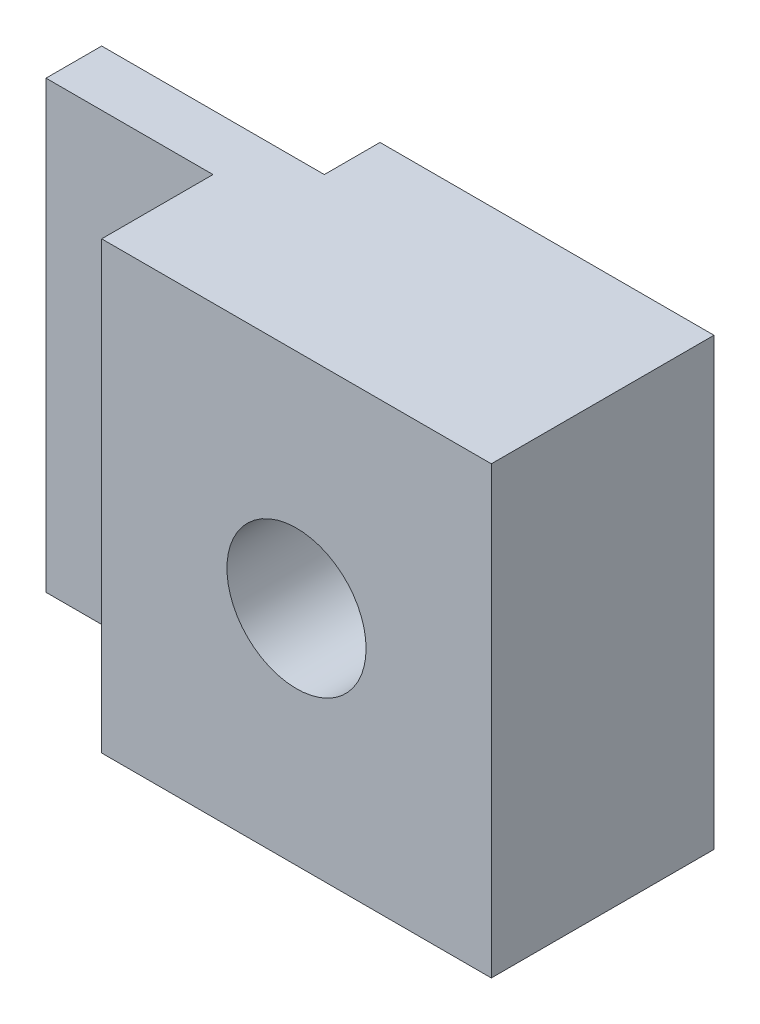
from build123d import *

# Parameters (mm, degrees)
SKETCH1_W             = 12
SKETCH1_H             = 8
BOSS_EXTRUDE1_DEPTH   = 2
SKETCH2_W             = 7
SKETCH2_H             = 8
BOSS_EXTRUDE2_DEPTH   = 2
SKETCH3_R             = 1.25
CUT_EXTRUDE1_DEPTH    = 10
CUT_EXTRUDE2_DEPTH    = 1
SKETCH5_W             = 2
SKETCH5_H             = 8
CUT_EXTRUDE3_DEPTH    = 7
MOVE_FACE1_BY         = 0.5
M3_TAPPED_HOLE4_D     = 2.5
M3_TAPPED_HOLE4_DEPTH = 7.5
M3_TAPPED_HOLE4_TIP   = 0.751075774


with BuildPart() as part:
    # Sketch1 → Boss-Extrude1 (new body)
    with BuildSketch(Plane.XY):
        with Locations((6, -4)):
            Rectangle(SKETCH1_W, SKETCH1_H)
    extrude(amount=BOSS_EXTRUDE1_DEPTH)

    # Sketch2 → Boss-Extrude2 (add)
    with BuildSketch(Plane.XY.offset(2)):
        with Locations((8.5, -4)):
            Rectangle(SKETCH2_W, SKETCH2_H)
    extrude(amount=BOSS_EXTRUDE2_DEPTH)

    # Sketch3 → Cut-Extrude1 (cut)
    with BuildSketch(Plane.XY.offset(4)):
        with Locations((8.5, -4)):
            Circle(SKETCH3_R)
    extrude(amount=-CUT_EXTRUDE1_DEPTH, mode=Mode.SUBTRACT)

    # Sketch4 → Cut-Extrude2 (cut)
    with BuildSketch(Plane(origin=(0, 0, 0), x_dir=(-1, 0, 0), z_dir=(0, 0, -1))):
        Polygon((0, -4), (0, 1.17366925), (-6, 1.17366925), (-6, -4), (-6, -6.5), (0, -6.5), align=None)
    extrude(amount=-CUT_EXTRUDE2_DEPTH, mode=Mode.SUBTRACT)

    # Sketch5 → Cut-Extrude3 (cut)
    with BuildSketch(Plane(origin=(0, 0, 0), x_dir=(-1, 0, 0), z_dir=(0, 0, -1))):
        with Locations((-1, -4)):
            Rectangle(SKETCH5_W, SKETCH5_H)
    extrude(amount=-CUT_EXTRUDE3_DEPTH, mode=Mode.SUBTRACT)

    # Move Face1: a curved face moved outward by 0.5
    add(Solid.thicken(part.faces().sort_by_distance((7.25, -4, 2))[0], MOVE_FACE1_BY))

    # M3 Tapped Hole4
    with Locations(Plane.XY.offset(4)):
        with Locations((8.5, -4)):
            Hole(M3_TAPPED_HOLE4_D / 2, depth=M3_TAPPED_HOLE4_DEPTH)
            with Locations((0, 0, -(M3_TAPPED_HOLE4_DEPTH + M3_TAPPED_HOLE4_TIP / 2))):  # 118° drill point
                Cone(0, M3_TAPPED_HOLE4_D / 2, M3_TAPPED_HOLE4_TIP, mode=Mode.SUBTRACT)


solid = part.part
